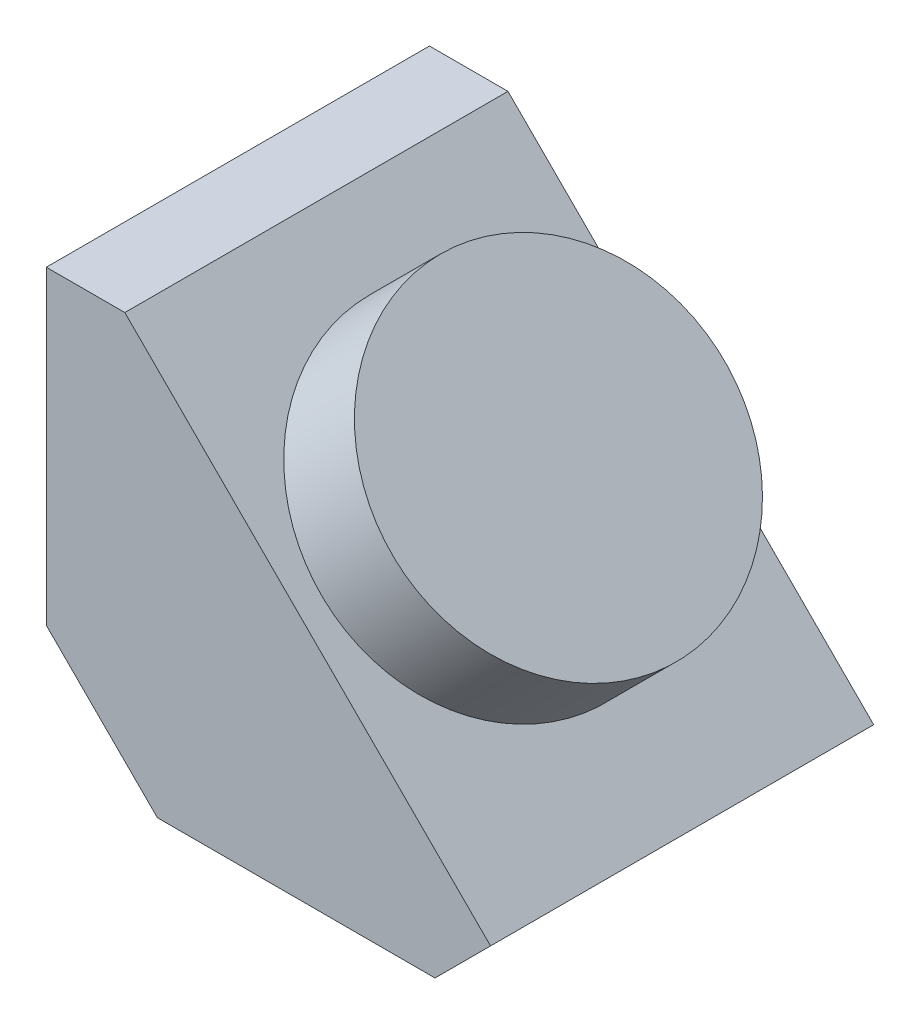
SolidWorks part; units mm, degrees
material "AL6061"
ref_plane "前视基准面" through (0, 0, 0) normal (0, 0, 1) x (1, 0, 0)
ref_plane "上视基准面" through (0, 0, 0) normal (0, 1, 0) x (1, 0, 0)
ref_plane "右视基准面" through (0, 0, 0) normal (1, 0, 0) x (0, 0, -1)
sketch "草图1" plane through (0, 0, 0) normal (0, 0, 1) x (1, 0, 0)
  line L0 (0, 0) -> (0, -90)
  line L1 (0, -90) -> (90, -90)
  line L2 (90, -90) -> (0, 0)
  dimension "D1" = 90
  dimension "D2" = 90
extrude "凸台-拉伸1" add sketch "草图1" along normal blind 69
chamfer "倒角1" distance 20 angle 45 1 edges at (0, -90, 34.5)
sketch "草图3" plane through (0, 0, 0) normal (0.7071, 0.7071, 0) x (0, 0, -1)
  line L0 (-34.5, 0) -> (-34.5, -63.6396) construction
  line L1 (-69, 0) -> (0, 0) construction
  line L2 (-34.5, -63.6396) -> (0, -63.6396) construction
  line L3 (0, -127.2792) -> (0, 0) construction
  circle A0 centre (-34.5, -63.6396) radius 30
  dimension "D1" = 60
extrude "凸台-拉伸2" add sketch "草图3" along normal blind 18
chamfer "倒角2" distance 20 angle 45 2 edges at (90, -90, 34.5) (0, 0, 34.5)
